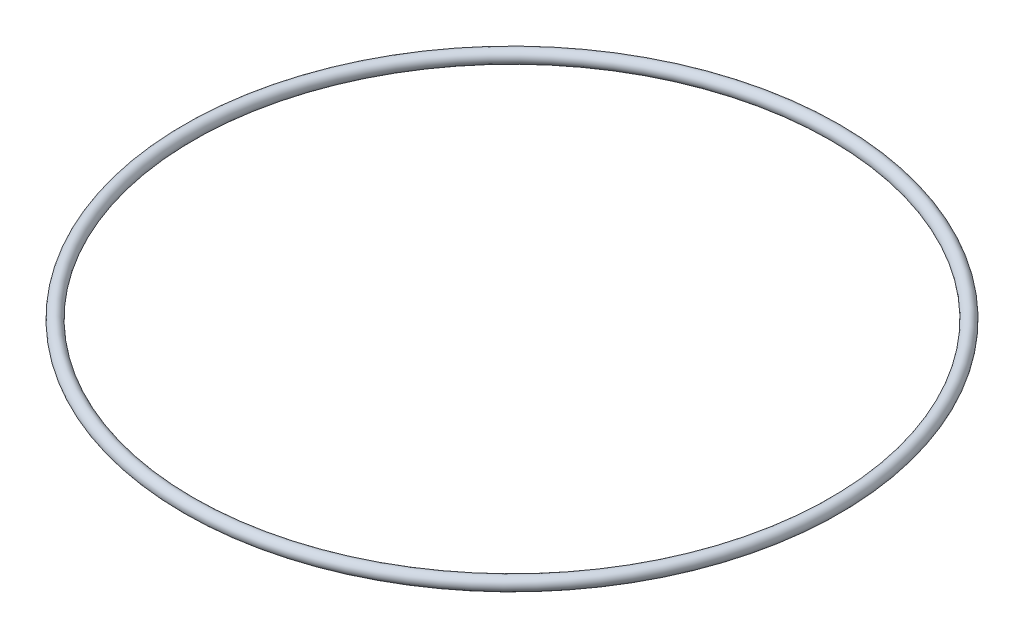
SolidWorks part; units mm, degrees
material "ABS"
ref_plane "Front Plane" through (0, 0, 0) normal (0, 0, 1) x (1, 0, 0)
ref_plane "Top Plane" through (0, 0, 0) normal (0, 1, 0) x (1, 0, 0)
ref_plane "Right Plane" through (0, 0, 0) normal (1, 0, 0) x (0, 0, -1)
sketch "Sketch1" plane through (0, 0, 0) normal (0, 0, 1) x (1, 0, 0)
  line L0 (0, 0) -> (0, 8.0454) construction
  circle A0 centre (-42.85, 0) radius 0.85
  dimension "D1" = 85.7
  dimension "D2" = 1.7
revolve "Revolve1" add sketch "Sketch1" angle 360 about L0
